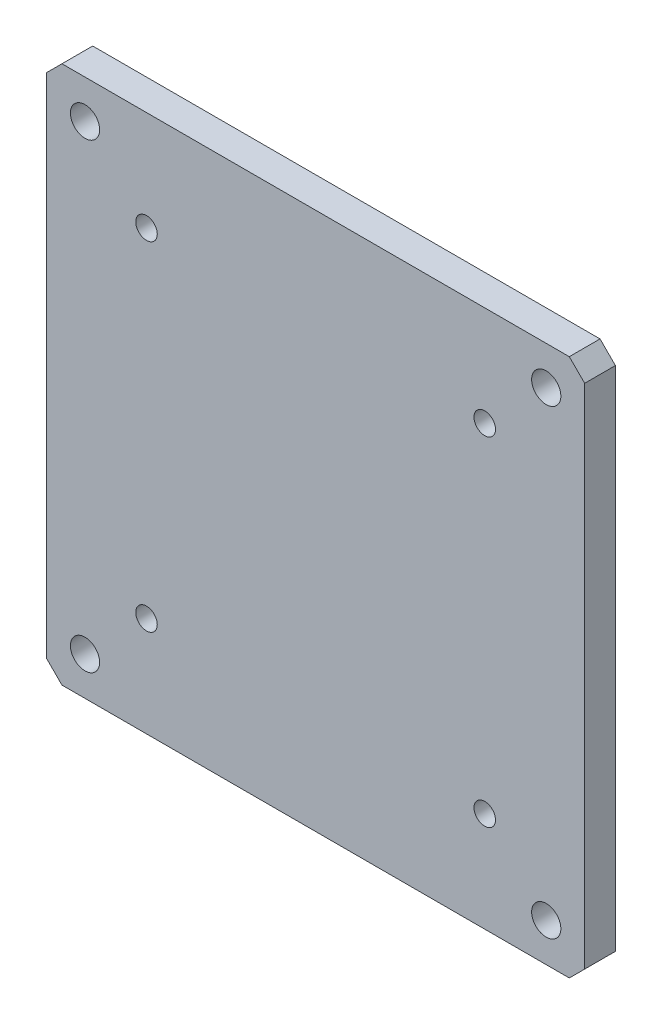
from build123d import *

# Parameters (mm, degrees)
SKETCH_1_W                  = 350
SKETCH_1_H                  = 350
EXTRUDE_1_DEPTH             = 20
HOLE_WIZARD_M16_1_D         = 14
HOLE_WIZARD_M16_1_DEPTH     = 42
HOLE_WIZARD_M16_1_TIP       = 4.206024333
HOLE_WIZARD_19_0_19_1_D     = 19
HOLE_WIZARD_19_0_19_1_DEPTH = 25
HOLE_WIZARD_19_0_19_1_TIP   = 5.708175881
CHAMFER_1_SIZE              = 10


with BuildPart() as part:
    # 草图1 → 凸台-拉伸1 (new body)
    with BuildSketch(Plane.XY):
        Rectangle(SKETCH_1_W, SKETCH_1_H)
    extrude(amount=EXTRUDE_1_DEPTH)

    # M16 螺纹孔1
    with Locations(Plane.XY.offset(20)):
        with Locations((110, 110), (-110, -110), (-110, 110), (110, -110)):
            Hole(HOLE_WIZARD_M16_1_D / 2, depth=HOLE_WIZARD_M16_1_DEPTH)
            with Locations((0, 0, -(HOLE_WIZARD_M16_1_DEPTH + HOLE_WIZARD_M16_1_TIP / 2))):  # 118° drill point
                Cone(0, HOLE_WIZARD_M16_1_D / 2, HOLE_WIZARD_M16_1_TIP, mode=Mode.SUBTRACT)

    # Ø19.0 (19) 直径孔1
    with Locations(Plane.XY.offset(20)):
        with Locations((150, 150), (-150, -150), (-150, 150), (150, -150)):
            Hole(HOLE_WIZARD_19_0_19_1_D / 2, depth=HOLE_WIZARD_19_0_19_1_DEPTH)
            with Locations((0, 0, -(HOLE_WIZARD_19_0_19_1_DEPTH + HOLE_WIZARD_19_0_19_1_TIP / 2))):  # 118° drill point
                Cone(0, HOLE_WIZARD_19_0_19_1_D / 2, HOLE_WIZARD_19_0_19_1_TIP, mode=Mode.SUBTRACT)

    # 倒角1
    chamfer_1_edges = [part.edges().sort_by_distance(p)[0] for p in [
        (175, -175, 10),
        (-175, -175, 10),
        (-175, 175, 10),
        (175, 175, 10),
    ]]
    chamfer(chamfer_1_edges, length=CHAMFER_1_SIZE)


solid = part.part
